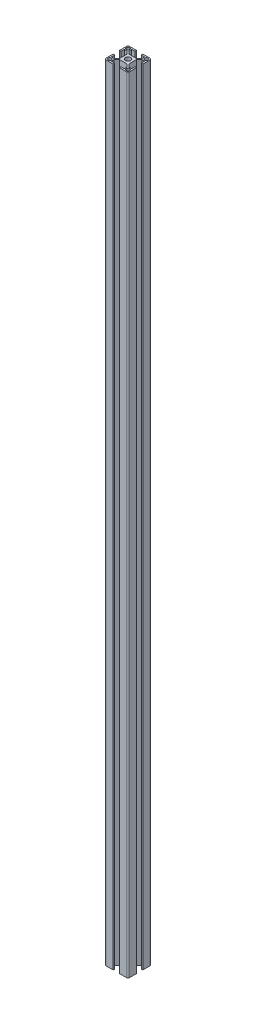
from build123d import *

# Parameters (mm, degrees)
SKETCH_1_R      = 2.1
SKETCH_1_R_2    = 3.4
EXTRUDE_1_DEPTH = 1000


with BuildPart() as part:
    # 草图1 → 拉伸1 (new body)
    with BuildSketch(Plane(origin=(0, 0, 0), x_dir=(1, 0, 0), z_dir=(0, 1, 0))):
        with BuildLine():
            Line((6.75, -28), (11, -28))
            Line((11, -28), (11, -30))
            Line((11, -30), (2, -30))
            ThreePointArc((2, -30), (0.585786438, -29.414213562), (0, -28))
            Line((0, -28), (0, -19))
            Line((0, -19), (2, -19))
            Line((2, -19), (2, -23.25))
            Line((2, -23.25), (5.335785999, -23.25))
            Line((5.335785999, -23.25), (9, -19.585785999))
            Line((9, -19.585785999), (9, -10.414214001))
            Line((9, -10.414214001), (5.335785999, -6.75))
            Line((5.335785999, -6.75), (2, -6.75))
            Line((2, -6.75), (2, -11))
            Line((2, -11), (0, -11))
            Line((0, -11), (0, -2))
            ThreePointArc((0, -2), (0.585786438, -0.585786438), (2, 0))
            Line((2, 0), (11, 0))
            Line((11, 0), (11, -2))
            Line((11, -2), (6.75, -2))
            Line((6.75, -2), (6.75, -5.335785999))
            Line((6.75, -5.335785999), (10.414214001, -9))
            Line((10.414214001, -9), (19.585785999, -9))
            Line((19.585785999, -9), (23.25, -5.335785999))
            Line((23.25, -5.335785999), (23.25, -2))
            Line((23.25, -2), (19, -2))
            Line((19, -2), (19, 0))
            Line((19, 0), (28, 0))
            ThreePointArc((28, 0), (29.414213562, -0.585786438), (30, -2))
            Line((30, -2), (30, -11))
            Line((30, -11), (28, -11))
            Line((28, -11), (28, -6.75))
            Line((28, -6.75), (24.664214001, -6.75))
            Line((24.664214001, -6.75), (21, -10.414214001))
            Line((21, -10.414214001), (21, -19.585785999))
            Line((21, -19.585785999), (24.664214001, -23.25))
            Line((24.664214001, -23.25), (28, -23.25))
            Line((28, -23.25), (28, -19))
            Line((28, -19), (30, -19))
            Line((30, -19), (30, -28))
            ThreePointArc((30, -28), (29.414213562, -29.414213562), (28, -30))
            Line((28, -30), (19, -30))
            Line((19, -30), (19, -28))
            Line((19, -28), (23.25, -28))
            Line((23.25, -28), (23.25, -24.664214001))
            Line((23.25, -24.664214001), (19.585785999, -21))
            Line((19.585785999, -21), (10.414214001, -21))
            Line((10.414214001, -21), (6.75, -24.664214001))
            Line((6.75, -24.664214001), (6.75, -28))
        make_face()
        with Locations(Location((3.375, -26.625, 0), (0, 0, 270))):
            Circle(SKETCH_1_R, mode=Mode.SUBTRACT)
        with Locations(Location((26.625, -26.625, 0), (0, 0, 270))):
            Circle(SKETCH_1_R, mode=Mode.SUBTRACT)
        with Locations(Location((15, -15, 0), (0, 0, 270))):
            Circle(SKETCH_1_R_2, mode=Mode.SUBTRACT)
        with Locations(Location((3.375, -3.375, 0), (0, 0, 270))):
            Circle(SKETCH_1_R, mode=Mode.SUBTRACT)
        with Locations(Location((26.625, -3.375, 0), (0, 0, 270))):
            Circle(SKETCH_1_R, mode=Mode.SUBTRACT)
    extrude(amount=EXTRUDE_1_DEPTH)


solid = part.part
